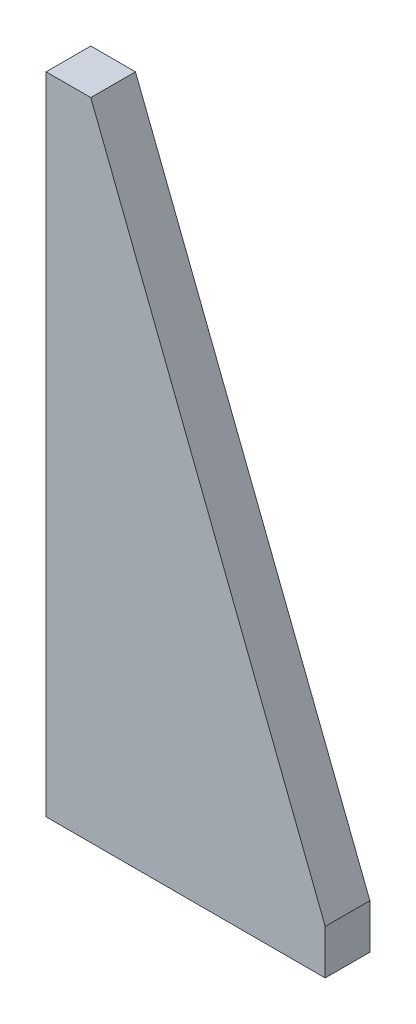
from build123d import *

# Parameters (mm, degrees)
BOSS_EXTRUDE1_DEPTH = 20


with BuildPart() as part:
    # Sketch1 → Boss-Extrude1 (new body)
    with BuildSketch(Plane.XY):
        Polygon((0, 0), (0, 289), (20, 289), (125, 20), (125, 0), align=None)
    extrude(amount=BOSS_EXTRUDE1_DEPTH)


solid = part.part
